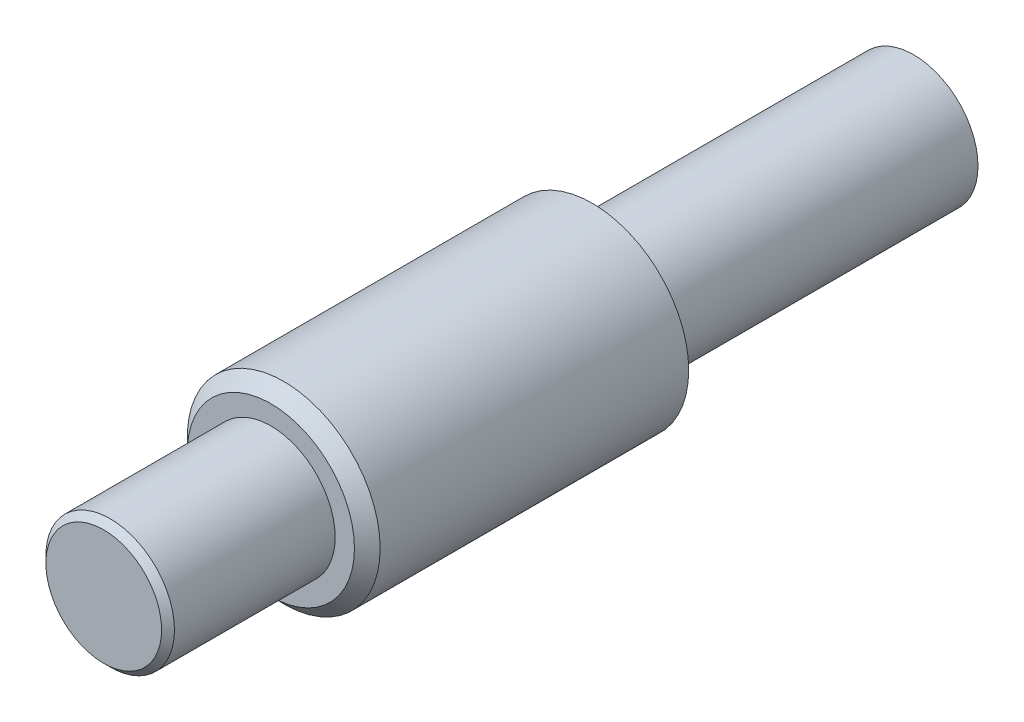
from build123d import *

# Parameters (mm, degrees)
SKETCH1_R           = 5
BOSS_EXTRUDE1_DEPTH = 25
SKETCH2_R           = 7.5
BOSS_EXTRUDE2_DEPTH = 8
SKETCH3_R           = 5
BOSS_EXTRUDE3_DEPTH = 30
SKETCH4_R           = 7.5
BOSS_EXTRUDE4_DEPTH = 17
CHAMFER1_SIZE       = 1
CHAMFER2_SIZE       = 0.5


with BuildPart() as part:
    # Sketch1 → Boss-Extrude1 (new body)
    with BuildSketch(Plane.XY):
        Circle(SKETCH1_R)
    extrude(amount=BOSS_EXTRUDE1_DEPTH)

    # Sketch2 → Boss-Extrude2 (add)
    with BuildSketch(Plane.XY.offset(25)):
        Circle(SKETCH2_R)
    extrude(amount=BOSS_EXTRUDE2_DEPTH)

    # Sketch3 → Boss-Extrude3 (add)
    with BuildSketch(Plane.XY.offset(33)):
        Circle(SKETCH3_R)
    extrude(amount=BOSS_EXTRUDE3_DEPTH)

    # Sketch4 → Boss-Extrude4 (add)
    with BuildSketch(Plane.XY.offset(33)):
        Circle(SKETCH4_R)
    extrude(amount=BOSS_EXTRUDE4_DEPTH)

    # Chamfer1
    chamfer1_edges = [part.edges().sort_by_distance(p)[0] for p in [
        (-7.5, 0, 50),
    ]]
    chamfer(chamfer1_edges, length=CHAMFER1_SIZE)

    # Chamfer2
    chamfer2_edges = [part.edges().sort_by_distance(p)[0] for p in [
        (-5, 0, 63),
    ]]
    chamfer(chamfer2_edges, length=CHAMFER2_SIZE)


solid = part.part
